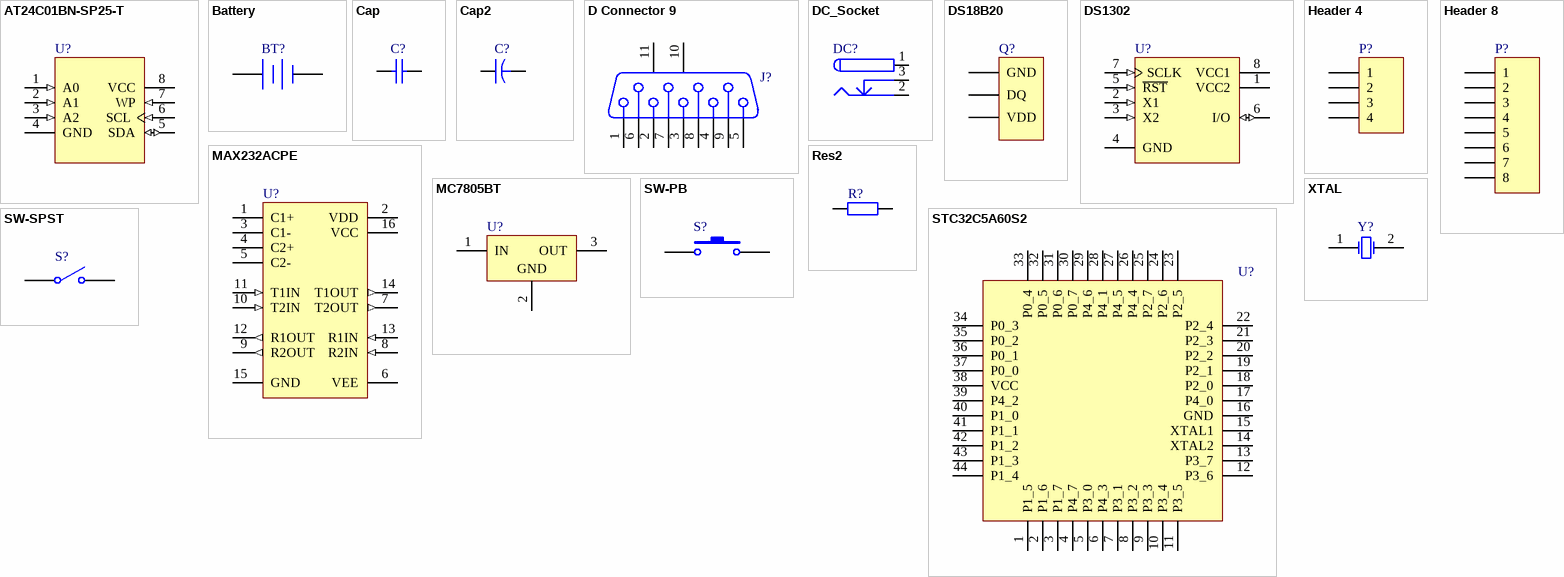
[diagram p0: symbols AT24C01BN-SP25-T to XTAL]
# Altium schematic symbol library MISC84364-7.SCHLIB: 17 symbols
Pins are listed as number, name and electrical type; pins without a type are passive.


## AT24C01BN-SP25-T
designator U?
1Kbit (128 x 8), 2-wire Bus Automotive Serial EEPROM with Write Protect, 2.5V, 8-Pin SOIC, Tape & Reel
footprint 8S1_N (SOIC, 8-Leads, Body 4.9x3.9mm, Pitch 1.27mm, IPC Medium Density)
footprint 8S1_L (SOIC, 8-Leads, Body 4.9x3.9mm, Pitch 1.27mm, IPC High Density)
footprint 8S1_M (SOIC, 8-Leads, Body 4.9x3.9mm, Pitch 1.27mm, IPC Low Density)
footprint DIP-8 (DIP; 8 Leads; Row Spacing 7.62 mm; Pitch 2.54 mm)
pins: 1 A0 (in), 2 A1 (in), 3 A2 (in), 4 GND (power), 5 SDA (io), 6 SCL (in), 7 WP (in), 8 VCC (power)

## Battery
designator BT?
Multicell Battery
footprint BAT-2 (Battery; 2 Leads)
pins: 1 +, 2 -

## Cap
designator C?
Capacitor
footprint RAD-0.3 (Radial Cap, Thru-Hole; 2 Leads; 0.3 in Pin Spacing)
simulation model CAP (Capacitor)
signal-integrity model Cap
footprint RAD-0.1 (Radial Cap, Thru-Hole; 2 Leads; 0.1 in Pin Spacing)
pins: 1, 2

## Cap2
designator C?
Capacitor
footprint CAPR5-4X5 (Capacitor; 2 Leads)
simulation model CAP (Capacitor)
signal-integrity model Cap
pins: 1, 2

## D Connector 9
designator J?
Receptacle Assembly, 9 Position, Right Angle
footprint DSUB1.385-2H9 (Connector; D Subminiature; 9 Position; Right Angle; Pitch 1.385 mm)
signal-integrity model Connector
pins: 1, 2, 3, 4, 5, 6, 7, 8, 9, 10 MH1, 11 MH2

## DC_Socket
designator DC?
footprint DC-002 (3.5X1.1mm)
footprint DC-003 (3.5X1.1mm)
footprint DC-003A (3.5X1.1mm)
footprint DC-005 (5.5X2.1mm)
footprint DC-012 (5.5X2.1mm)
footprint DC-031A (3.5X1.3mm)
footprint DC-050 (5.5X2.1mm)
pins: 1 (power), 2 (power), 3 (power)

## DS18B20
designator Q?
数字温度计
footprint TO92A (92晶体管)
footprint TO92B (92晶体管)
footprint HDR1X1
footprint HDR1X3 (Connector; Header; 3 Position)
pins: 1 GND, 2 DQ, 3 VDD

## DS1302
designator U?
Trickle Charge Timekeeping Chip
footprint DIP8 (DIP; 8 Leads; Row Spacing 7.62 mm; Pitch 2.54 mm)
pins: 1 VCC2 (power), 2 X1 (in), 3 X2 (in), 4 GND (power), 5 ~{RST} (in), 6 I/O (io), 7 SCLK (in), 8 VCC1 (power)

## Header 4
designator P?
Header, 4-Pin
footprint HDR1X4 (Connector; Header; 4 Position)
signal-integrity model Connector
pins: 1, 2, 3, 4

## Header 8
designator P?
Header, 8-Pin
footprint HDR1X8 (Connector; Header; 8 Position)
signal-integrity model Connector
pins: 1, 2, 3, 4, 5, 6, 7, 8

## MAX232ACPE
designator U?
+5V Powered, Multi-Channel RS-232 Driver/Receiver
footprint PE16A (DIP; 16 Leads; Row Spacing 7.62 mm; Pitch 2.54 mm)
pins: 1 C1+, 2 VDD (power), 3 C1-, 4 C2+, 5 C2-, 6 VEE (power), 7 T2OUT (out), 8 R2IN (in), 9 R2OUT (out), 10 T2IN (in), 11 T1IN (in), 12 R1OUT (out), 13 R1IN (in), 14 T1OUT (out), 15 GND (power), 16 VCC (power)

## MC7805BT
designator U?
3-Terminal Positive Fixed Voltage Regulator
footprint 221A-04 (TO, Thru-Hole, Vertical, Heatsink Mounted; 3 In-Line Leads; Pitch 2.54 mm)
pins: 1 IN (power), 2 GND (power), 3 OUT (power)

## Res2
designator R?
Resistor
footprint AXIAL-0.4 (Axial Device, Thru-Hole; 2 Leads; 0.4 in Pin Spacing)
simulation model RESISTOR (Resistor)
signal-integrity model Res
pins: 1, 2

## STC32C5A60S2
designator U?
STC32C5A60S2
footprint LQFP48 7X7
pins: 1 P1_5, 2 P1_6, 3 P1_7, 4 P4_7, 5 P3_0, 6 P4_3, 7 P3_1, 8 P3_2, 9 P3_3, 10 P3_4, 11 P3_5, 12 P3_6, 13 P3_7, 14 XTAL2, 15 XTAL1, 16 GND, 17 P4_0, 18 P2_0, 19 P2_1, 20 P2_2, 21 P2_3, 22 P2_4, 23 P2_5, 24 P2_6, 25 P2_7, 26 P4_4, 27 P4_5, 28 P4_1, 29 P4_6, 30 P0_7, 31 P0_6, 32 P0_5, 33 P0_4, 34 P0_3, 35 P0_2, 36 P0_1, 37 P0_0, 38 VCC, 39 P4_2, 40 P1_0, 41 P1_1, 42 P1_2, 43 P1_3, 44 P1_4

## SW-PB
designator S?
Switch
footprint SPST-2 (Switch; 2 Leads)
pins: 1, 2

## SW-SPST
designator S?
Single-Pole, Single-Throw Switch
footprint SPST-2 (Switch; 2 Leads)
pins: 1 COMMON, 2 NO

## XTAL
designator Y?
Crystal Oscillator
footprint R38 (Crystal, Thru-Hole; 2 Leads; Body 3.1 x 8.2 mm (Dia.xH))
simulation model XTAL (Spice Subcircuit)
pins: 1 OSC1, 2 OSC2